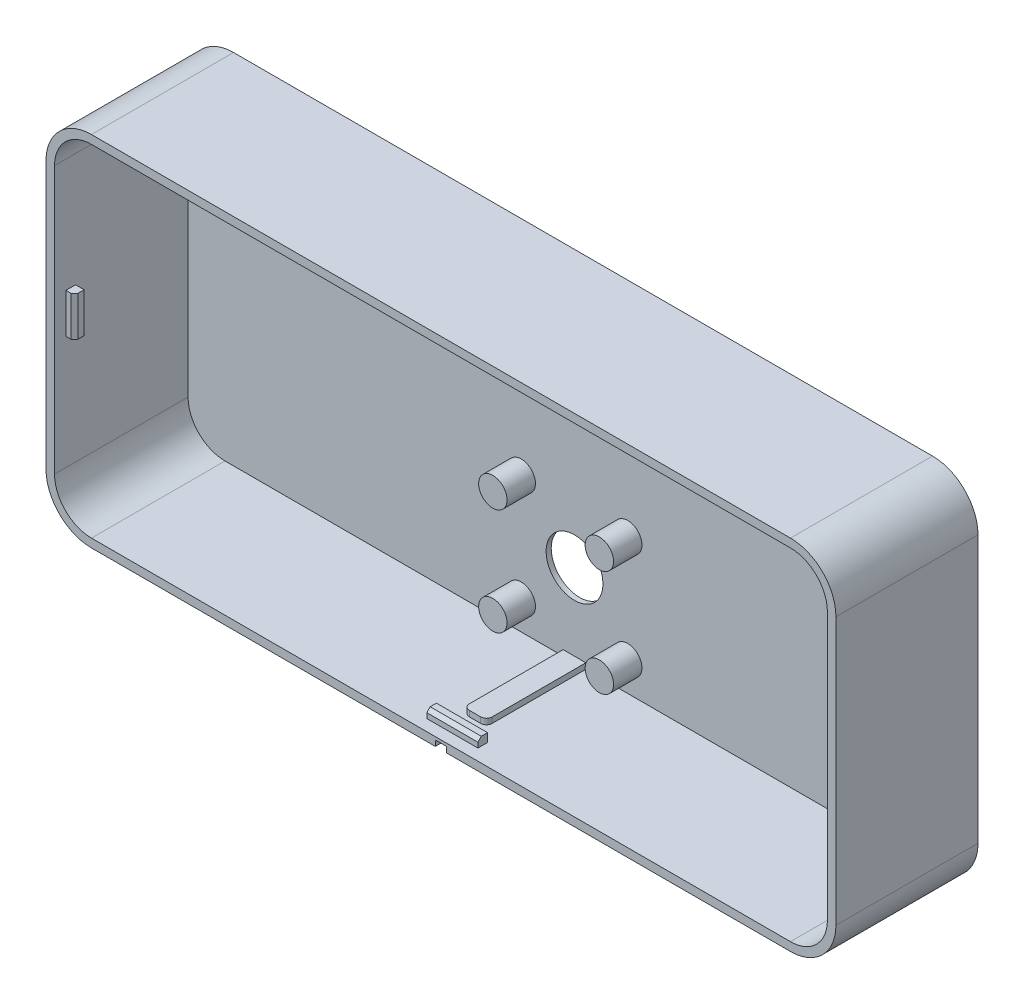
SolidWorks part; units mm, degrees
ref_plane "Front Plane" through (0, 0, 0) normal (0, 0, 1) x (1, 0, 0)
ref_plane "Top Plane" through (0, 0, 0) normal (0, 1, 0) x (1, 0, 0)
ref_plane "Right Plane" through (0, 0, 0) normal (1, 0, 0) x (0, 0, -1)
other "Configuration Table"
sketch "Sketch1" plane through (0, 0, 0) normal (0, 0, 1) x (1, 0, 0)
  line L1 (-61.5, 31.5) -> (61.5, 31.5)
  line L2 (-69.5, 23.5) -> (-69.5, -23.5)
  line L3 (-61.5, -31.5) -> (61.5, -31.5)
  line L4 (69.5, 23.5) -> (69.5, -23.5)
  line L5 (-69.5, 31.5) -> (69.5, -31.5) construction
  line L6 (-69.5, -31.5) -> (69.5, 31.5) construction
  arc A0 (-69.5, -23.5) -> (-61.5, -31.5) centre (-61.5, -23.5) ccw
  arc A1 (61.5, -31.5) -> (69.5, -23.5) centre (61.5, -23.5) ccw
  arc A2 (61.5, 31.5) -> (69.5, 23.5) centre (61.5, 23.5) cw
  arc A3 (-61.5, 31.5) -> (-69.5, 23.5) centre (-61.5, 23.5) ccw
  point P0 (0, 0)
  dimension "D3" = 8
  dimension "D1" = 139
  dimension "D2" = 63
extrude "Boss-Extrude1" add sketch "Sketch1" along normal blind 25
shell "Shell1" thickness 1.5
sketch "Sketch2" plane through (0, 30, 0) normal (0, -1, 0) x (-1, 0, 0)
  line L0 (61.5, -25) -> (-61.5, -25) construction
  line L15 (4.5, -23) -> (-4.5, -23)
  line L16 (4.5, -23) -> (4.5, -21.3)
  line L17 (4.5, -21.3) -> (-4.5, -21.3)
  line L18 (-4.5, -23) -> (-4.5, -21.3)
  line L19 (4.5, -23) -> (-4.5, -21.3) construction
  line L20 (4.5, -21.3) -> (-4.5, -23) construction
  point P5 (0, -22.15)
  dimension "D3" = 1.7
  dimension "D5" = 2
  dimension "D6" = 9
extrude "Boss-Extrude2" add sketch "Sketch2" along normal blind 1.5
chamfer "Chamfer1" distance 0.6 angle 45 1 edges at (0, 28.5, 23)
mirror "Mirror1" about plane through (0, 0, 0) normal (0, 1, 0) of "Chamfer1", "Boss-Extrude2"
sketch "Sketch3" plane through (0, -30, 0) normal (0, 1, 0) x (1, 0, 0)
  line L0 (-61.5, -1.5) -> (61.5, -1.5) construction
  line L1 (-2, -1.5) -> (2, -1.5)
  line L2 (-2, -1.5) -> (-2, -19)
  line L3 (-2, -19) -> (2, -19)
  line L4 (2, -1.5) -> (2, -19)
  line L6 (61.5, -25) -> (-61.5, -25) construction
  dimension "D1" = 2
  dimension "D2" = 4
  dimension "D3" = 6
extrude "Boss-Extrude3" add sketch "Sketch3" along normal blind 1
sketch "Sketch6" plane through (0, 0, 0) normal (0, 0, -1) x (-1, 0, 0)
  line L0 (61.5, -31.5) -> (-61.5, -31.5) construction
  circle A0 centre (0, -15.5) radius 10.15
  dimension "D1" = 20.3
  dimension "D2" = 16
extrude "Cut-Extrude3" cut sketch "Sketch6" against normal blind 0.6
sketch "Sketch10" plane through (0, 0, 0.6) normal (0, 0, -1) x (-1, 0, 0)
  circle A0 centre (0, -15.5) radius 5
  dimension "D1" = 10
extrude "Cut-Extrude4" cut sketch "Sketch10" against normal through all
sketch "Sketch11" plane through (0, 0, 0.6) normal (0, 0, -1) x (-1, 0, 0)
  circle A0 centre (0, -15.5) radius 7
  circle A2 centre (0, -15.5) radius 8
  dimension "D1" = 16
  dimension "D2" = 14
extrude "Boss-Extrude5" add sketch "Sketch11" along normal blind 0.6
sketch "Sketch13" plane through (0, 0, 1.5) normal (0, 0, 1) x (1, 0, 0)
  line L0 (0, -15.5) -> (0, 0) construction
  line L1 (0, -15.5) -> (-9.3692, -6.1308) construction
  circle A0 centre (0, -15.5) radius 13.25 construction
  circle A1 centre (-9.3692, -6.1308) radius 2.5
  circle A2 centre (9.3692, -6.1308) radius 2.5
  circle A3 centre (9.3692, -24.8692) radius 2.5
  circle A4 centre (-9.3692, -24.8692) radius 2.5
  circle A5 centre (0, -15.5) radius 5 construction
  point P16 (0, -15.5)
  dimension "D1" = 26.5
  dimension "D3" = 5
  dimension "D2" = 45
  dimension "D4" = 4
extrude "Boss-Extrude6" add sketch "Sketch13" along normal blind 5
sketch "Sketch15" plane through (0, 0, 6.5) normal (0, 0, 1) x (1, 0, 0)
  circle A0 centre (9.3692, -6.1308) radius 0.5
  circle A1 centre (-9.3692, -6.1308) radius 0.5
  circle A2 centre (-9.3692, -24.8692) radius 0.5
  circle A3 centre (9.3692, -24.8692) radius 0.5
  dimension "D1" = 1
extrude "Cut-Extrude5" cut sketch "Sketch15" against normal through all from offset 2 offset against normal yes
sketch "Sketch16" plane through (0, -31.5, 0) normal (0, -1, 0) x (-1, 0, 0)
  line L1 (1, 29.0822) -> (-1, 29.0822)
  line L2 (1, 29.0822) -> (1, -29.0822)
  line L3 (1, -29.0822) -> (-1, -29.0822)
  line L4 (-1, 29.0822) -> (-1, -29.0822)
  line L5 (1, 29.0822) -> (-1, -29.0822) construction
  line L6 (1, -29.0822) -> (-1, 29.0822) construction
  point P0 (0, 0)
  dimension "D1" = 2
extrude "Cut-Extrude6" cut sketch "Sketch16" against normal blind 1
fillet "Fillet2" radius 0.1 4 edges at (-7, -15.5, 0) (-8, -15.5, 0) (-7, -15.5, 0.6) (-8, -15.5, 0.6)
sketch "Sketch17" plane through (0, 0, 0) normal (0, 0, -1) x (-1, 0, 0)
  circle A0 centre (0, -15.5) radius 15.5
  circle A1 centre (0, -15.5) radius 10.15
  circle A2 centre (-9.3692, -6.1308) radius 0.5
  circle A3 centre (9.3692, -6.1308) radius 0.5
  circle A4 centre (9.3692, -24.8692) radius 0.5
  circle A5 centre (-9.3692, -24.8692) radius 0.5
  dimension "D1" = 31
  dimension "D2" = 1
  dimension "D3" = 20.3
extrude "Boss-Extrude7" add sketch "Sketch17" along normal blind 1.2
sketch "Sketch18" plane through (0, -31.5, 0) normal (0, -1, 0) x (-1, 0, 0)
  line L1 (1, 0) -> (-1, 0)
  line L2 (1, 0) -> (1, 1.6262)
  line L3 (1, 1.6262) -> (-1, 1.6262)
  line L4 (-1, 0) -> (-1, 1.6262)
  dimension "D1" = 2
extrude "Cut-Extrude7" cut sketch "Sketch18" against normal blind 1
fillet "Fillet3" radius 0.5 1 edges at (0, 0, 0)
fillet "Fillet4" radius 1 2 edges at (-2, -29.5, 19) (2, -29.5, 19)
sketch "Sketch19" plane through (-68, 0, 0) normal (1, 0, 0) x (0, 0, -1)
  line L0 (-25, 23.5) -> (-25, -23.5) construction
  line L1 (-23, 3.5) -> (-21.3, 3.5)
  line L2 (-23, 3.5) -> (-23, -3.5)
  line L3 (-23, -3.5) -> (-21.3, -3.5)
  line L4 (-21.3, 3.5) -> (-21.3, -3.5)
  line L5 (-23, 3.5) -> (-21.3, -3.5) construction
  line L6 (-23, -3.5) -> (-21.3, 3.5) construction
  point P0 (-22.15, 0)
  dimension "D1" = 1.7
  dimension "D2" = 2
  dimension "D3" = 7
extrude "Boss-Extrude8" add sketch "Sketch19" along normal blind 1.5
chamfer "Chamfer2" distance 0.6 angle 45 1 edges at (-66.5, 0, 23)
mirror "Mirror2" about plane through (0, 0, 0) normal (1, 0, 0) of "Chamfer2", "Boss-Extrude8"
fillet "Fillet5" radius 0.2 2 edges at (1, -30.5, 11.9) (-1, -30.5, 11.9)
